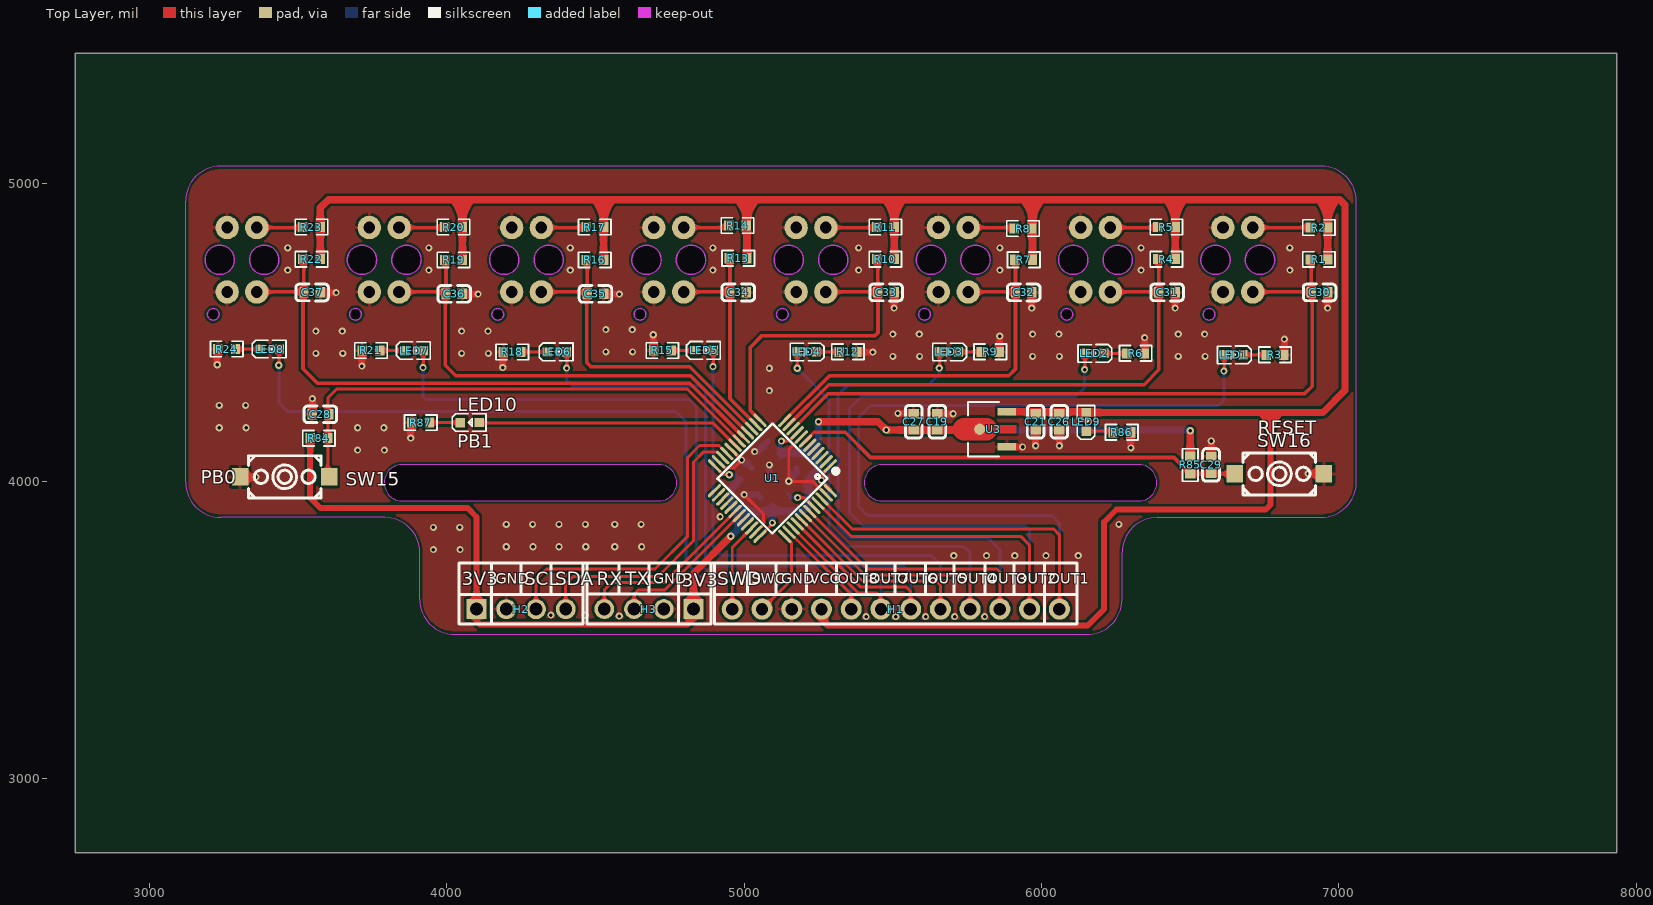
[diagram p0: Top Layer view]
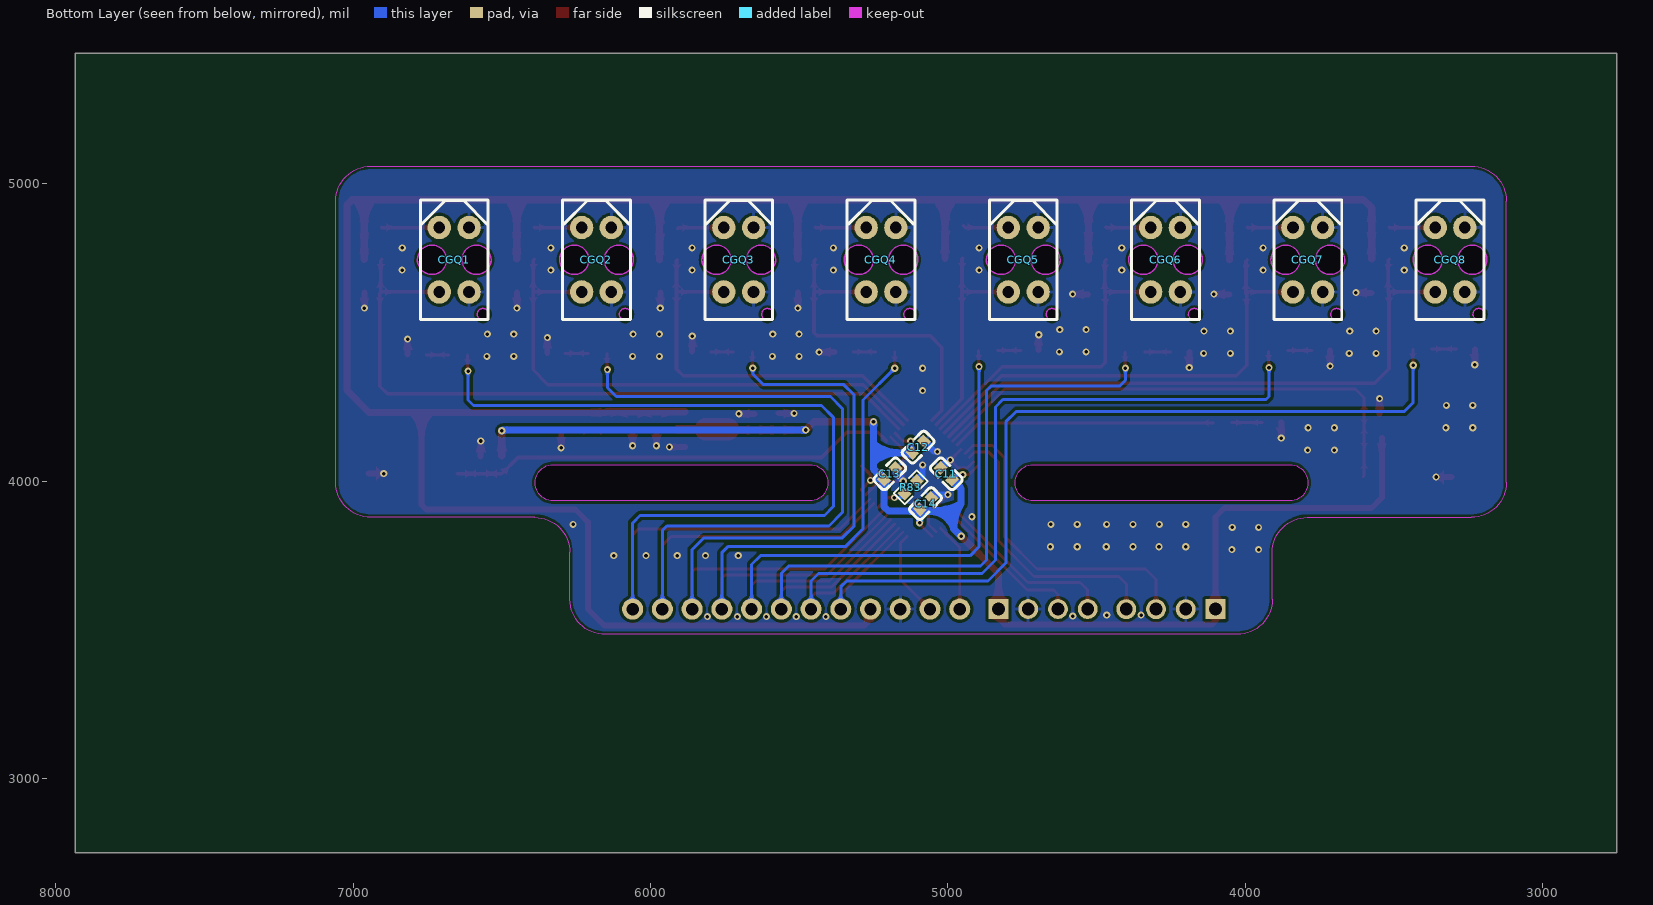
[diagram p1: Bottom Layer view, seen from below]
# Altium PCB MISC51279.pcbdoc (part 1 of 3)
Units mil, origin at the board's own origin, x right, y up, seen from the top; angles counter-clockwise.
Board outline 5185 x 2690 mil, 2 copper layers (Top Layer, Bottom Layer), stack 62.206 mil thick; 72 components, 47 nets, 221 pads, 129 vias.

## Layer stack, top to bottom
Top Solder Mask Layer: solder mask 0.394, Dk 3.3
Top Layer: signal copper 1.379
Dielectric1: surface 59.449, FR4, Dk 4.5
Bottom Layer: signal copper 1.378
Bottom Solder Mask Layer: solder mask 0.394, Dk 3.3

## Board outline
7935,2750 2750,2750 2750,5440 7935,5440
cut-out: 3850.31,4056.06 ccw(c3850.31,3995.04) 3789.29,3995.04 ccw(c3850.31,3995.04) 3850.31,3934.02 4712.52,3934.02 ccw(c4712.52,3995.04) 4773.54,3995.04 ccw(c4712.52,3995.04) 4712.52,4056.06 3850.31,4056.06
cut-out: 5464.49,4056.06 ccw(c5464.49,3995.04) 5403.46,3995.04 ccw(c5464.49,3995.04) 5464.49,3934.02 6326.69,3934.02 ccw(c6326.69,3995.04) 6387.72,3995.04 ccw(c6326.69,3995.04) 6326.69,4056.06 5464.49,4056.06

## Design rules (kind name [scope] priority, off if disabled: settings)
BoardOutlineClearance copperThickness2oz_1 [All] p2 off: genericclearance=7.99 ignorepadtopadclearanceinfootprint=FALSE except(0: Arc-SplitContinuation Track-SplitContinuation SMDPad-SplitContinuation THPad-SplitContinuation Via-SplitContinuation Fill-SplitContinuation Region-SplitContinuation Poly-SplitContinuation Text-SplitContinuation Hole-SplitContinuation; 5.98: Arc-CutoutEdge Track-CutoutEdge SMDPad-CutoutEdge THPad-CutoutEdge Via-CutoutEdge Text-CutoutEdge; 6.9: Hole-OutlineEdge Hole-CutoutEdge; 10: Poly-OutlineEdge Poly-CutoutEdge; 11.81: Arc-OutlineEdge Track-OutlineEdge SMDPad-OutlineEdge THPad-OutlineEdge Via-OutlineEdge Fill-OutlineEdge Region-OutlineEdge Text-OutlineEdge Fill-CutoutEdge Region-CutoutEdge)
BoardOutlineClearance Plane_innerPlane_1 [All] p4 off: genericclearance=4.02 ignorepadtopadclearanceinfootprint=FALSE except(0: Arc-SplitContinuation Track-SplitContinuation SMDPad-SplitContinuation THPad-SplitContinuation Via-SplitContinuation Fill-SplitContinuation Region-SplitContinuation Poly-SplitContinuation Text-SplitContinuation Hole-SplitContinuation; 5.98: Arc-CutoutEdge Track-CutoutEdge SMDPad-CutoutEdge THPad-CutoutEdge Via-CutoutEdge Text-CutoutEdge; 6.9: Hole-OutlineEdge Hole-CutoutEdge; 10: Poly-OutlineEdge Poly-CutoutEdge; 11.81: Arc-OutlineEdge Track-OutlineEdge SMDPad-OutlineEdge THPad-OutlineEdge Via-OutlineEdge Fill-OutlineEdge Region-OutlineEdge Text-OutlineEdge Fill-CutoutEdge Region-CutoutEdge)
BoardOutlineClearance Copper_copperRegion_1 [All] p6 off: genericclearance=4.02 ignorepadtopadclearanceinfootprint=FALSE except(0: Arc-SplitContinuation Track-SplitContinuation SMDPad-SplitContinuation THPad-SplitContinuation Via-SplitContinuation Fill-SplitContinuation Region-SplitContinuation Poly-SplitContinuation Text-SplitContinuation Hole-SplitContinuation; 5.98: Arc-CutoutEdge Track-CutoutEdge SMDPad-CutoutEdge THPad-CutoutEdge Via-CutoutEdge Text-CutoutEdge; 6.9: Hole-OutlineEdge Hole-CutoutEdge; 10: Poly-OutlineEdge Poly-CutoutEdge; 11.81: Arc-OutlineEdge Track-OutlineEdge SMDPad-OutlineEdge THPad-OutlineEdge Via-OutlineEdge Fill-OutlineEdge Region-OutlineEdge Text-OutlineEdge Fill-CutoutEdge Region-CutoutEdge)
BoardOutlineClearance copperThickness1oz_1 [All] p8: genericclearance=4.02 ignorepadtopadclearanceinfootprint=FALSE except(0: Arc-SplitContinuation Track-SplitContinuation SMDPad-SplitContinuation THPad-SplitContinuation Via-SplitContinuation Fill-SplitContinuation Region-SplitContinuation Poly-SplitContinuation Text-SplitContinuation Hole-SplitContinuation; 5.98: Arc-CutoutEdge Track-CutoutEdge SMDPad-CutoutEdge THPad-CutoutEdge Via-CutoutEdge Text-CutoutEdge; 6.9: Hole-OutlineEdge Hole-CutoutEdge; 10: Poly-OutlineEdge Poly-CutoutEdge; 11.81: Arc-OutlineEdge Track-OutlineEdge SMDPad-OutlineEdge THPad-OutlineEdge Via-OutlineEdge Fill-OutlineEdge Region-OutlineEdge Text-OutlineEdge Fill-CutoutEdge Region-CutoutEdge)
Clearance copperThickness2oz [All] p1 off: gap=7.99 ignorepadtopadclearanceinfootprint=FALSE except(5.98: SMDPad-Track SMDPad-SMDPad THPad-Track SMDPad-THPad THPad-THPad Track-Via SMDPad-Via THPad-Via Via-Via Fill-SMDPad Region-SMDPad Fill-THPad Region-THPad Fill-Via Region-Via Fill-Fill Fill-Region Region-Region Arc-Track Arc-SMDPad Arc-THPad Arc-Via Fill-Arc Region-Arc Arc-Arc Text-Track SMDPad-Text Text-THPad Text-Via Fill-Text Region-Text Arc-Text Text-Text; 6.9: Hole-Track Hole-SMDPad Hole-THPad Hole-Via Fill-Hole Region-Hole Hole-Arc Hole-Text; 10: Poly-Track Poly-SMDPad Poly-THPad Poly-Via Poly-Fill Poly-Region Poly-Poly Poly-Arc Poly-Text Poly-Hole; 11.81: Fill-Track Region-Track)
Clearance Plane_innerPlane [All] p3 off: gap=4.02 ignorepadtopadclearanceinfootprint=FALSE except(5.98: SMDPad-Track SMDPad-SMDPad THPad-Track SMDPad-THPad THPad-THPad Track-Via SMDPad-Via THPad-Via Via-Via Fill-SMDPad Region-SMDPad Fill-THPad Region-THPad Fill-Via Region-Via Fill-Fill Fill-Region Region-Region Arc-Track Arc-SMDPad Arc-THPad Arc-Via Fill-Arc Region-Arc Arc-Arc Text-Track SMDPad-Text Text-THPad Text-Via Fill-Text Region-Text Arc-Text Text-Text; 6.9: Hole-Track Hole-SMDPad Hole-THPad Hole-Via Fill-Hole Region-Hole Hole-Arc Hole-Text; 10: Poly-Track Poly-SMDPad Poly-THPad Poly-Via Poly-Fill Poly-Region Poly-Poly Poly-Arc Poly-Text Poly-Hole; 11.81: Fill-Track Region-Track)
Clearance Copper_copperRegion [All] p5 off: gap=4.02 ignorepadtopadclearanceinfootprint=FALSE except(5.98: SMDPad-Track SMDPad-SMDPad THPad-Track SMDPad-THPad THPad-THPad Track-Via SMDPad-Via THPad-Via Via-Via Fill-SMDPad Region-SMDPad Fill-THPad Region-THPad Fill-Via Region-Via Fill-Fill Fill-Region Region-Region Arc-Track Arc-SMDPad Arc-THPad Arc-Via Fill-Arc Region-Arc Arc-Arc Text-Track SMDPad-Text Text-THPad Text-Via Fill-Text Region-Text Arc-Text Text-Text; 6.9: Hole-Track Hole-SMDPad Hole-THPad Hole-Via Fill-Hole Region-Hole Hole-Arc Hole-Text; 10: Poly-Track Poly-SMDPad Poly-THPad Poly-Via Poly-Fill Poly-Region Poly-Poly Poly-Arc Poly-Text Poly-Hole; 11.81: Fill-Track Region-Track)
Clearance copperThickness1oz [All] p7: gap=4.02 ignorepadtopadclearanceinfootprint=FALSE except(5.98: SMDPad-Track SMDPad-SMDPad THPad-Track SMDPad-THPad THPad-THPad Track-Via SMDPad-Via THPad-Via Via-Via Fill-SMDPad Region-SMDPad Fill-THPad Region-THPad Fill-Via Region-Via Fill-Fill Fill-Region Region-Region Arc-Track Arc-SMDPad Arc-THPad Arc-Via Fill-Arc Region-Arc Arc-Arc Text-Track SMDPad-Text Text-THPad Text-Via Fill-Text Region-Text Arc-Text Text-Text; 6.9: Hole-Track Hole-SMDPad Hole-THPad Hole-Via Fill-Hole Region-Hole Hole-Arc Hole-Text; 10: Poly-Track Poly-SMDPad Poly-THPad Poly-Via Poly-Fill Poly-Region Poly-Poly Poly-Arc Poly-Text Poly-Hole; 11.81: Fill-Track Region-Track)
DiffPairsRouting differentialPair [All] p1: maxlimit=6 minlimit=6 mostfreqgap=6 toplayer_minwidth=5 toplayer_prefwidth=10 toplayer_maxwidth=100 toplayer_mingap=6 toplayer_prefgap=6 toplayer_maxgap=6 bottomlayer_minwidth=5 bottomlayer_prefwidth=10 bottomlayer_maxwidth=100 bottomlayer_mingap=6 bottomlayer_prefgap=6 bottomlayer_maxgap=6 maxuncoupledlength=10
HoleToHoleClearance otherClearance [All] p1: gap=11.81 allowstackedmicrovias=TRUE
Length netLength [All] p1: minlimit=0 maxlimit=0
PasteMaskExpansion pasteMaskExpansion [All] p1: expansion=0
PlaneConnect innerPlane [All] p1: planeconnectstyle=Relief reliefexpansion=20 reliefentries=4 reliefconductorwidth=10 reliefairgap=10
PolygonConnect copperRegion [All] p1: connectstyle=Relief reliefconductorwidth=10 reliefentries=4 polygonreliefangle="90 Angle" airgapwidth=10 via.connectstyle=Relief via.reliefconductorwidth=10 via.reliefentries=4 via.polygonreliefangle="90 Angle" via.airgapwidth=10
RoutingVias viaSize [All] p1: holewidth=12.01 width=24.02 viastyle="Through Hole" minholewidth=11.81 minwidth=19.68 maxholewidth=248.03 maxwidth=393.7
SolderMaskExpansion solderMaskExpansion [IsVia] p1: expansion=-1000 istentingtop=TRUE
SolderMaskExpansion solderMaskExpansion [All] p2: expansion=2 istentingtop=FALSE
Width copperThickness2oz_2 [All] p1 off: maxlimit=100 minlimit=8 preferedwidth=10
Width copperThickness1oz_2 [All] p2: maxlimit=100 minlimit=5 preferedwidth=10

## Components (designator, comment, footprint, x,y, rotation, side; value= is the part's Value field where it differs from the comment)
C11 "100nF" C0603 5005,4025 r225 bottom
C12 "100nF" C0603 5100,4115 r315 bottom
C13 "100nF" C0603 5195,4025 r315 bottom
C14 "100nF" C0603 5075,3925 r315 bottom
C19 "100nF" C0603 5650,4199.99 r270 top
C21 "100nF" C0603 5980,4200 r90 top
C26 "10uF" C0603 6060,4200 r270 top
C27 "10uF" C0603 5570,4199.99 r90 top
C28 "100nF" C0603 3575,4225 r0 top
C29 "100nF" C0603 6570,4055 r270 top
C30 "100nF" C0603 6935,4635 r0 top
C31 "100nF" C0603 6422.19,4635 r0 top
C32 "100nF" C0603 5940,4635 r0 top
C33 "100nF" C0603 5477.19,4635 r0 top
C34 "100nF" C0603 4980,4635 r0 top
C35 "100nF" C0603 4500,4630 r0 top
C36 "100nF" C0603 4025,4630 r0 top
C37 "100nF" C0603 3547.19,4635 r0 top
CGQ1 "TCRT5000L" OPTO-TH_TCRT5000L 6660,4745 r90 bottom
CGQ2 "TCRT5000L" OPTO-TH_TCRT5000L 6181.61,4745 r90 bottom
CGQ3 "TCRT5000L" OPTO-TH_TCRT5000L 5703.22,4745 r90 bottom
CGQ4 "TCRT5000L" OPTO-TH_TCRT5000L 5224.83,4745 r90 bottom
CGQ5 "TCRT5000L" OPTO-TH_TCRT5000L 4746.44,4745 r90 bottom
CGQ6 "TCRT5000L" OPTO-TH_TCRT5000L 4268.04,4745 r90 bottom
CGQ7 "TCRT5000L" OPTO-TH_TCRT5000L 3789.65,4745 r90 bottom
CGQ8 "TCRT5000L" OPTO-TH_TCRT5000L 3311.26,4745 r90 bottom
H1 "" HDR-TH_12P-P2.54-V-F 5510,3570 r180 top
H2 "" HDR-TH_4P-P2.54-V-F 4250,3570 r0 top
H3 "" HDR-TH_4P-P2.54-V-F 4679.69,3570.18 r180 top
LED1 "NCD0603R1" LED0603-RD_RED 6646.27,4425.21 r180 top
LED2 "NCD0603R1" LED0603-RD_RED 6177.54,4430.21 r180 top
LED3 "NCD0603R1" LED0603-RD_RED 5688.81,4435.21 r180 top
LED4 "NCD0603R1" LED0603-RD_RED 5210.08,4435.21 r180 top
LED5 "NCD0603R1" LED0603-RD_RED 4865,4440 r0 top
LED6 "NCD0603R1" LED0603-RD_RED 4370,4435 r0 top
LED7 "NCD0603R1" LED0603-RD_RED 3889.83,4439.58 r0 top
LED8 "NCD0603R1" LED0603-RD_RED 3404.83,4444.58 r0 top
LED9 "NCD0603R1" LED0603-RD_RED 6150,4200 r90 top
LED10 "NCD0603R1" LED0603-RD_RED 4077.21,4197.37 r0 top
R1 "10kΩ" R0603 6932.81,4746.18 r0 top
R2 "1kΩ" R0603 6932.81,4853.42 r0 top
R3 "1kΩ" R0603 6785.08,4425.21 r0 top
R4 "10kΩ" R0603 6420,4746.97 r0 top
R5 "1kΩ" R0603 6420,4855 r0 top
R6 "1kΩ" R0603 6316.36,4430.21 r0 top
R7 "10kΩ" R0603 5940,4745 r0 top
R8 "1kΩ" R0603 5937.81,4850 r0 top
R9 "1kΩ" R0603 5827.63,4435.21 r0 top
R10 "10kΩ" R0603 5475,4746.97 r0 top
R11 "1kΩ" R0603 5475,4855 r0 top
R12 "1kΩ" R0603 5348.9,4435.21 r0 top
R13 "10kΩ" R0603 4980,4750 r0 top
R14 "1kΩ" R0603 4977.81,4860 r0 top
R15 "1kΩ" R0603 4725,4440 r180 top
R16 "10kΩ" R0603 4497.81,4744.47 r0 top
R17 "1kΩ" R0603 4497.81,4855 r0 top
R18 "1kΩ" R0603 4220,4435 r180 top
R19 "10kΩ" R0603 4022.81,4744.47 r0 top
R20 "1kΩ" R0603 4022.81,4855 r0 top
R21 "1kΩ" R0603 3745,4440 r180 top
R22 "10kΩ" R0603 3545,4746.97 r0 top
R23 "1kΩ" R0603 3545,4855 r0 top
R24 "1kΩ" R0603 3259.83,4444.58 r180 top
R83 "1kΩ" R0603 5125,3980 r315 bottom
R84 "10K" R0603 3570,4145 r180 top
R85 "10K" R0603 6500,4055 r90 top
R86 "1kΩ" R0603 6270,4165 r0 top
R87 "1kΩ" R0603 3912.21,4197.37 r180 top
SW15 "K2-1107ST-A4DW-06" KEY-SMD_L6.2-W3.6-LS8.0 3455,4015 r180 top
SW16 "K2-1107ST-A4DW-06" KEY-SMD_L6.2-W3.6-LS8.0 6800,4025 r0 top
U1 "STM32F103C8T6" LQFP-48_L7.0-W7.0-P0.50-LS9.0-BL 5095,4010 r135 top
U3 "CJA1117B-3.3" SOT-89-3_L4.5-W2.5-P1.50-LS4.2-BR 5830,4174.99 r0 top

## Footprints (in the part's own frame and the unit in brackets; to place one, negate y for a bottom-side part, rotate by r counter-clockwise, add the part's x,y. Pads: shape width x height; smd on the part's side, far side on the other; paste and mask are expansions set on the pad)
C0603 [mm]
  rect 0.8x0.9 smd: 1(-0.7,0) 2(0.7,0)
  silkscreen extent -1.39,-0.71 1.39,0.71
HDR-TH_4P-P2.54-V-F [mm]
  rect 1.7x1.7 hole 1.1: 1(-3.81,0)
  round 1.7 hole 1.1: 2(-1.27,0) 3(1.27,0) 4(3.81,0)
  silkscreen extent -5.29,-1.27 5.29,1.27
HDR-TH_12P-P2.54-V-F [mm]
  round 1.8 hole 1.05: 1(-13.97,0) 2(-11.43,0) 3(-8.89,0) 4(-6.35,0) 5(-3.81,0) 6(-1.27,0) 7(1.27,0) 8(3.81,0) 9(6.35,0) 10(8.89,0) 11(11.43,0) 12(13.97,0)
  silkscreen extent -15.49,-1.25 15.49,1.25
KEY-SMD_L6.2-W3.6-LS8.0 [mm]
  rect 1.4x1.5 smd: 1(-3.8,0) 2(3.8,0)
  silkscreen extent -3.1,-1.8 3.1,1.8
LED0603-RD_RED [mm]
  rect 0.8x0.8 smd: 1(-0.8,-0.003) 2(0.8,0.003)
  silkscreen extent -1.49,-0.75 1.39,0.76
LQFP-48_L7.0-W7.0-P0.50-LS9.0-BL [mm]
  oval 0.27x1.5 smd paste+0 mask+0.05: 1(-2.75,-4.25) 2(-2.25,-4.25) 3(-1.75,-4.25) 4(-1.25,-4.25) 5(-0.75,-4.25) 6(-0.25,-4.25) 7(0.25,-4.25) 8(0.75,-4.25) 9(1.25,-4.25) 10(1.75,-4.25) 11(2.25,-4.25) 12(2.75,-4.25) 25(2.75,4.25) 26(2.25,4.25) 27(1.75,4.25) 28(1.25,4.25) 29(0.75,4.25) 30(0.25,4.25) 31(-0.25,4.25) 32(-0.75,4.25) 33(-1.25,4.25) 34(-1.75,4.25) 35(-2.25,4.25) 36(-2.75,4.25)
  oval 1.5x0.27 smd paste+0 mask+0.05: 13(4.25,-2.75) 14(4.25,-2.25) 15(4.25,-1.75) 16(4.25,-1.25) 17(4.25,-0.75) 18(4.25,-0.25) 19(4.25,0.25) 20(4.25,0.75) 21(4.25,1.25) 22(4.25,1.75) 23(4.25,2.25) 24(4.25,2.75) 37(-4.25,2.75) 38(-4.25,2.25) 39(-4.25,1.75) 40(-4.25,1.25) 41(-4.25,0.75) 42(-4.25,0.25) 43(-4.25,-0.25) 44(-4.25,-0.75) 45(-4.25,-1.25) 46(-4.25,-1.75) 47(-4.25,-2.25) 48(-4.25,-2.75)
  silkscreen extent -3.59,-4.46 3.3,3.34
OPTO-TH_TCRT5000L [mm]
  round 2 hole 1: 1(-2.751,1.27) 2(-2.751,-1.27) 3(2.751,1.27) 4(2.751,-1.27)
  Board Outline Layer circle w0.003: c-0.008,1.897 r1.25
  Board Outline Layer circle w0.003: c-0.008,-1.902 r1.25
  Board Outline Layer circle w0.003: c-4.658,-2.454 r0.5
  Board Outline Layer region: -0.008,3.147 -0.55,3.024 -0.985,2.677 -1.226,2.176 -1.226,1.619 -0.985,1.118 -0.55,0.771 -0.008,0.647 -0.008,0.647 0.535,0.771 0.97,1.118 1.211,1.619 1.211,2.176 0.97,2.677 0.535,3.024 -0.008,3.147
  Board Outline Layer region: -0.008,3.147 -0.164,3.138 -0.318,3.108 -0.468,3.06 -0.61,2.993 -0.742,2.909 -0.863,2.809 -0.971,2.694 -1.063,2.567 -1.139,2.43 -1.196,2.284 -1.235,2.132 -1.255,1.976 -1.255,1.819 -1.235,1.663 -1.196,1.511 -1.139,1.365 -1.063,1.228 -0.971,1.101 -0.863,0.986 -0.742,0.886 -0.61,0.802 -0.468,0.735 -0.318,0.687 -0.164,0.657 -0.008,0.647 0.149,0.657 0.303,0.687 0.453,0.735 0.595,0.802 0.727,0.886 0.848,0.986 0.956,1.101 1.048,1.228 1.123,1.365 1.181,1.511 1.22,1.663 1.24,1.819 1.24,1.976 1.22,2.132 1.181,2.284 1.123,2.43 1.048,2.567 0.956,2.694 0.848,2.809 0.727,2.909 0.595,2.993 0.453,3.06 0.303,3.108 0.149,3.138
  Board Outline Layer region: -0.008,-0.652 -0.55,-0.776 -0.985,-1.123 -1.226,-1.624 -1.226,-2.181 -0.985,-2.682 -0.55,-3.029 -0.008,-3.152 -0.008,-3.152 0.535,-3.029 0.97,-2.682 1.211,-2.181 1.211,-1.624 0.97,-1.123 0.535,-0.776 -0.008,-0.652
  Board Outline Layer region: -0.008,-0.652 -0.164,-0.662 -0.318,-0.692 -0.468,-0.74 -0.61,-0.807 -0.742,-0.891 -0.863,-0.991 -0.971,-1.106 -1.063,-1.233 -1.139,-1.37 -1.196,-1.516 -1.235,-1.668 -1.255,-1.824 -1.255,-1.981 -1.235,-2.137 -1.196,-2.289 -1.139,-2.435 -1.063,-2.572 -0.971,-2.699 -0.863,-2.814 -0.742,-2.914 -0.61,-2.998 -0.468,-3.065 -0.318,-3.113 -0.164,-3.143 -0.008,-3.152 0.149,-3.143 0.303,-3.113 0.453,-3.065 0.595,-2.998 0.727,-2.914 0.848,-2.814 0.956,-2.699 1.048,-2.572 1.123,-2.435 1.181,-2.289 1.22,-2.137 1.24,-1.981 1.24,-1.824 1.22,-1.668 1.181,-1.516 1.123,-1.37 1.048,-1.233 0.956,-1.106 0.848,-0.991 0.727,-0.891 0.595,-0.807 0.453,-0.74 0.303,-0.692 0.149,-0.662
  Board Outline Layer region: -4.658,-1.954 -4.875,-2.003 -5.049,-2.142 -5.146,-2.342 -5.146,-2.565 -5.049,-2.765 -4.875,-2.904 -4.658,-2.954 -4.658,-2.954 -4.441,-2.904 -4.267,-2.765 -4.171,-2.565 -4.171,-2.342 -4.267,-2.142 -4.441,-2.003 -4.658,-1.954
  Board Outline Layer region: -4.658,-1.954 -4.756,-1.963 -4.85,-1.992 -4.936,-2.038 -5.012,-2.1 -5.074,-2.176 -5.12,-2.262 -5.149,-2.356 -5.158,-2.454 -5.149,-2.551 -5.12,-2.645 -5.074,-2.731 -5.012,-2.807 -4.936,-2.869 -4.85,-2.916 -4.756,-2.944 -4.658,-2.954 -4.561,-2.944 -4.467,-2.916 -4.381,-2.869 -4.305,-2.807 -4.243,-2.731 -4.196,-2.645 -4.168,-2.551 -4.158,-2.454 -4.168,-2.356 -4.196,-2.262 -4.243,-2.176 -4.305,-2.1 -4.381,-2.038 -4.467,-1.992 -4.561,-1.963
  Multi-Layer board cut-out: -0.008,3.147 -0.55,3.024 -0.985,2.677 -1.226,2.176 -1.226,1.619 -0.985,1.118 -0.55,0.771 -0.008,0.647 -0.008,0.647 0.535,0.771 0.97,1.118 1.211,1.619 1.211,2.176 0.97,2.677 0.535,3.024 -0.008,3.147
  Multi-Layer board cut-out: -0.008,-0.652 -0.55,-0.776 -0.985,-1.123 -1.226,-1.624 -1.226,-2.181 -0.985,-2.682 -0.55,-3.029 -0.008,-3.152 -0.008,-3.152 0.535,-3.029 0.97,-2.682 1.211,-2.181 1.211,-1.624 0.97,-1.123 0.535,-0.776 -0.008,-0.652
  Multi-Layer board cut-out: -4.658,-1.954 -4.875,-2.003 -5.049,-2.142 -5.146,-2.342 -5.146,-2.565 -5.049,-2.765 -4.875,-2.904 -4.658,-2.954 -4.658,-2.954 -4.441,-2.904 -4.267,-2.765 -4.171,-2.565 -4.171,-2.342 -4.267,-2.142 -4.441,-2.003 -4.658,-1.954
  silkscreen extent -5.11,-2.9 5.09,2.9
R0603 [mil]
  rect 31.75x34.02 smd paste-3937.01 mask+2: 1(-29.66,0) 2(29.66,0)
  silkscreen extent -55,-26 55,26
SOT-89-3_L4.5-W2.5-P1.50-LS4.2-BR [mm]
  rect 1.575x0.672 smd: 1(1.356,-1.5) 3(1.356,1.5)
  round 0.95 smd: 2(-0.966,0)
  Top Layer region: -2.283,0.95 -0.429,0.95 -0.384,0.949 -0.34,0.946 -0.296,0.94 -0.252,0.933 -0.208,0.924 -0.165,0.912 -0.123,0.899 -0.081,0.884 -0.04,0.866 0,0.847 0.04,0.826 0.078,0.803 0.115,0.779 0.151,0.752 0.185,0.724 0.219,0.695 0.251,0.664 0.281,0.631 0.31,0.597 0.337,0.562 0.362,0.525 0.386,0.488 0.408,0.449 0.428,0.409 0.447,0.33 2.144,0.33 2.144,-0.33 0.447,-0.33 0.428,-0.409 0.408,-0.449 0.386,-0.488 0.362,-0.526 0.337,-0.562 0.31,-0.597 0.281,-0.631 0.251,-0.664 0.219,-0.695 0.185,-0.725 0.151,-0.753 0.115,-0.779 0.078,-0.804 0.04,-0.827 0,-0.848 -0.04,-0.867 -0.081,-0.884 -0.123,-0.899 -0.165,-0.913 -0.208,-0.924 -0.252,-0.934 -0.296,-0.941 -0.34,-0.946 -0.384,-0.949 -0.429,-0.95 -2.283,-0.95 -2.328,-0.949 -2.372,-0.946 -2.416,-0.941 -2.46,-0.934 -2.504,-0.924 -2.547,-0.913 -2.589,-0.899 -2.631,-0.884 -2.672,-0.867 -2.713,-0.848 -2.752,-0.827 -2.79,-0.804 -2.827,-0.779 -2.863,-0.753 -2.898,-0.725 -2.931,-0.695 -2.963,-0.664 -2.993,-0.631 -3.022,-0.597 -3.049,-0.562 -3.075,-0.526 -3.098,-0.488 -3.12,-0.449 -3.141,-0.409 -3.159,-0.369 -3.175,-0.327 -3.189,-0.285 -3.202,-0.242 -3.212,-0.199 -3.22,-0.155 -3.227,-0.111 -3.231,-0.067 -3.233,-0.022 -3.233,0.022 -3.231,0.067 -3.227,0.111 -3.22,0.155 -3.212,0.199 -3.202,0.242 -3.189,0.285 -3.175,0.327 -3.159,0.369 -3.141,0.409 -3.12,0.449 -3.098,0.488 -3.075,0.525 -3.049,0.562 -3.022,0.597 -2.993,0.631 -2.963,0.664 -2.931,0.695 -2.898,0.724 -2.863,0.752 -2.827,0.779 -2.79,0.803 -2.752,0.826 -2.713,0.847 -2.672,0.866 -2.631,0.884 -2.589,0.899 -2.547,0.912 -2.504,0.924 -2.46,0.933 -2.416,0.94 -2.372,0.946 -2.328,0.949
  silkscreen extent -1.95,-2.33 0.7,2.33

## Via types
v1: diameter 24.02, hole 12, Top Layer to Bottom Layer, 129 vias